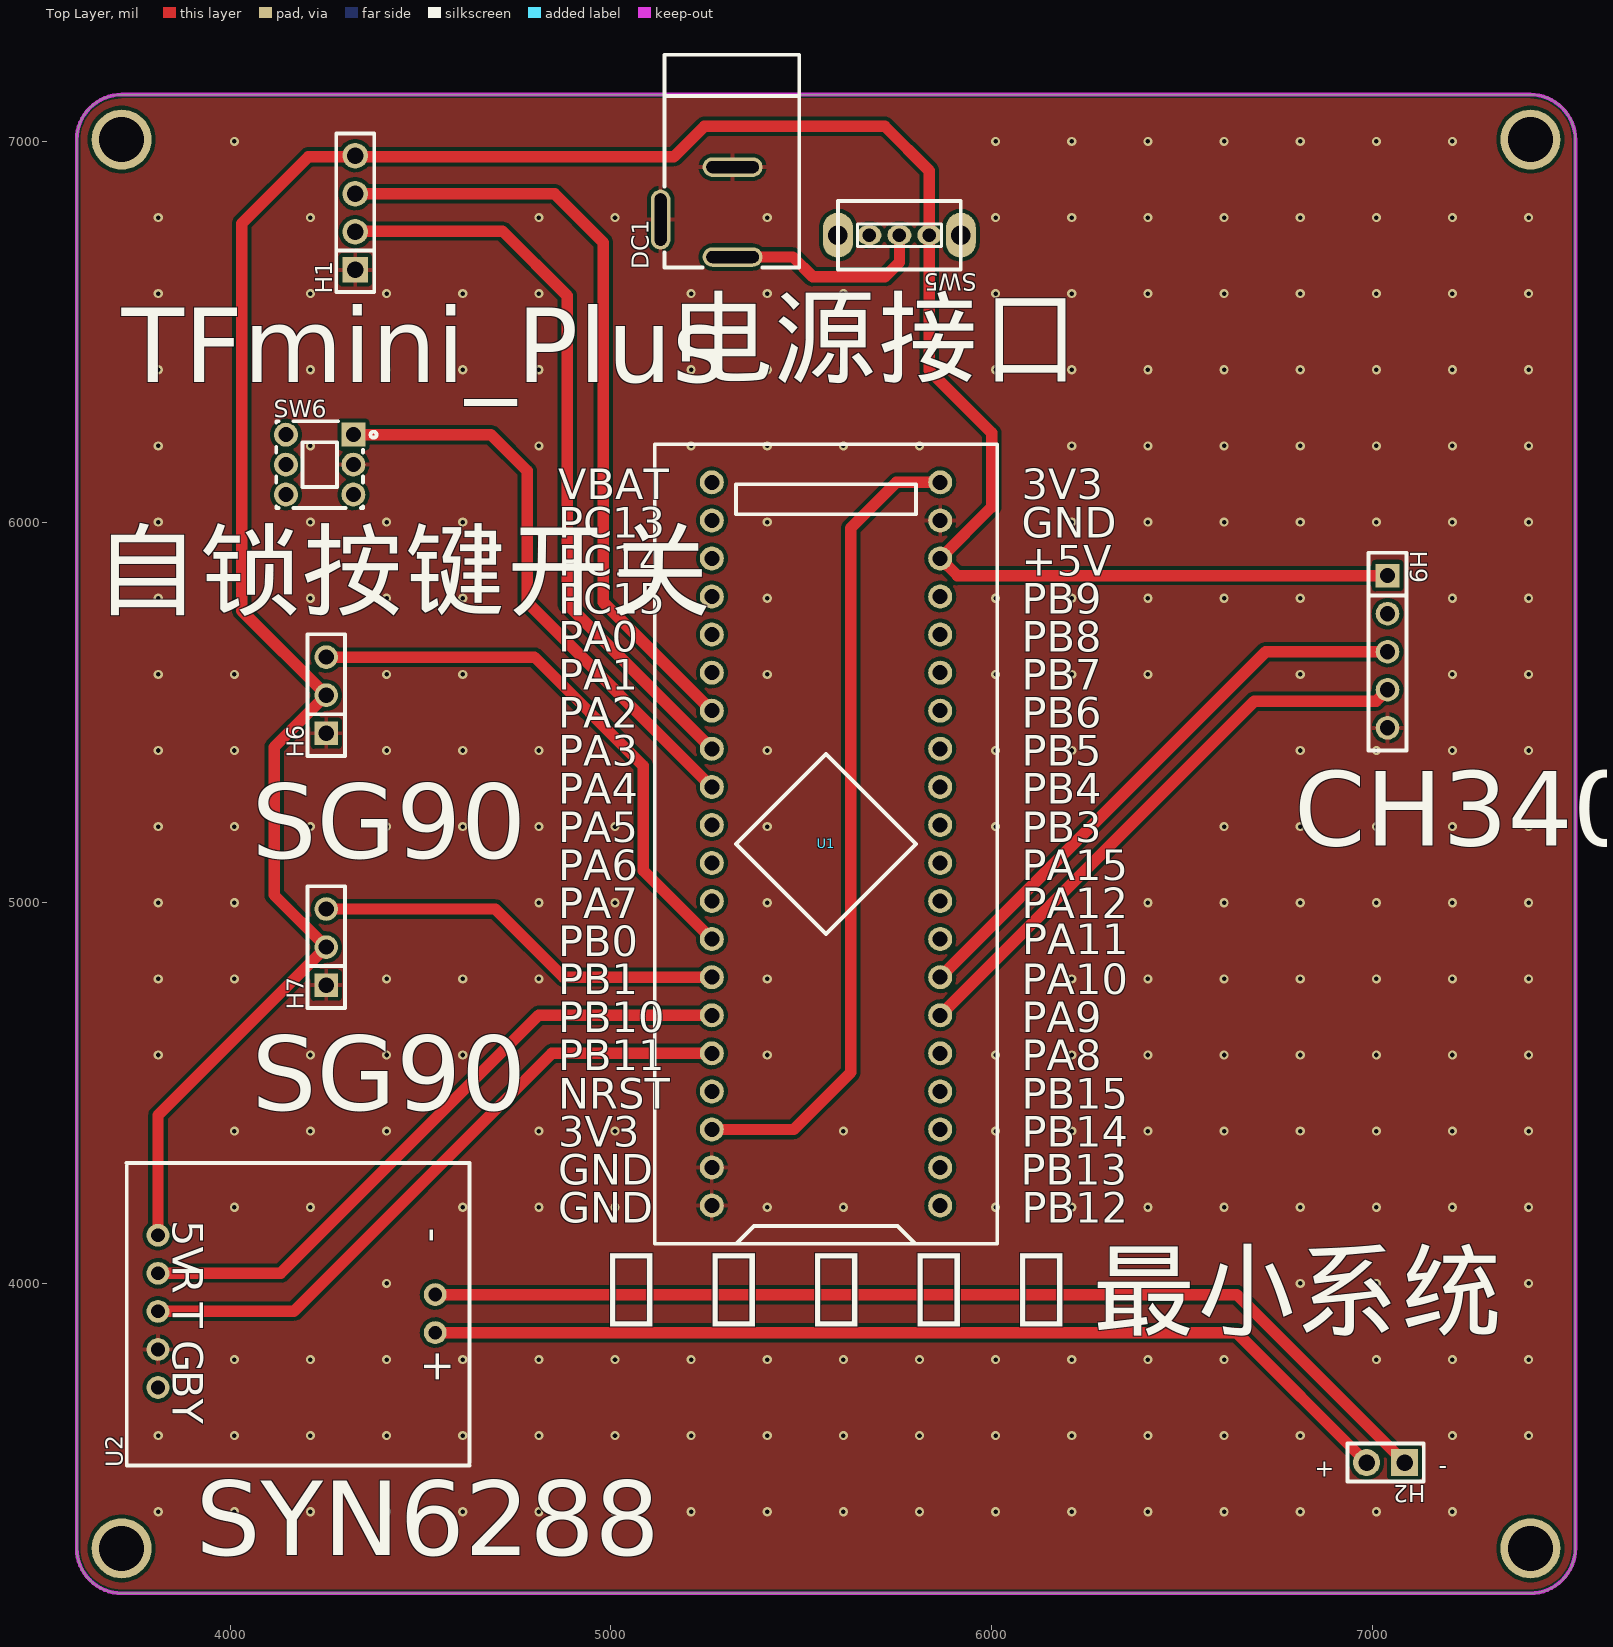
[diagram p0: Top Layer view]
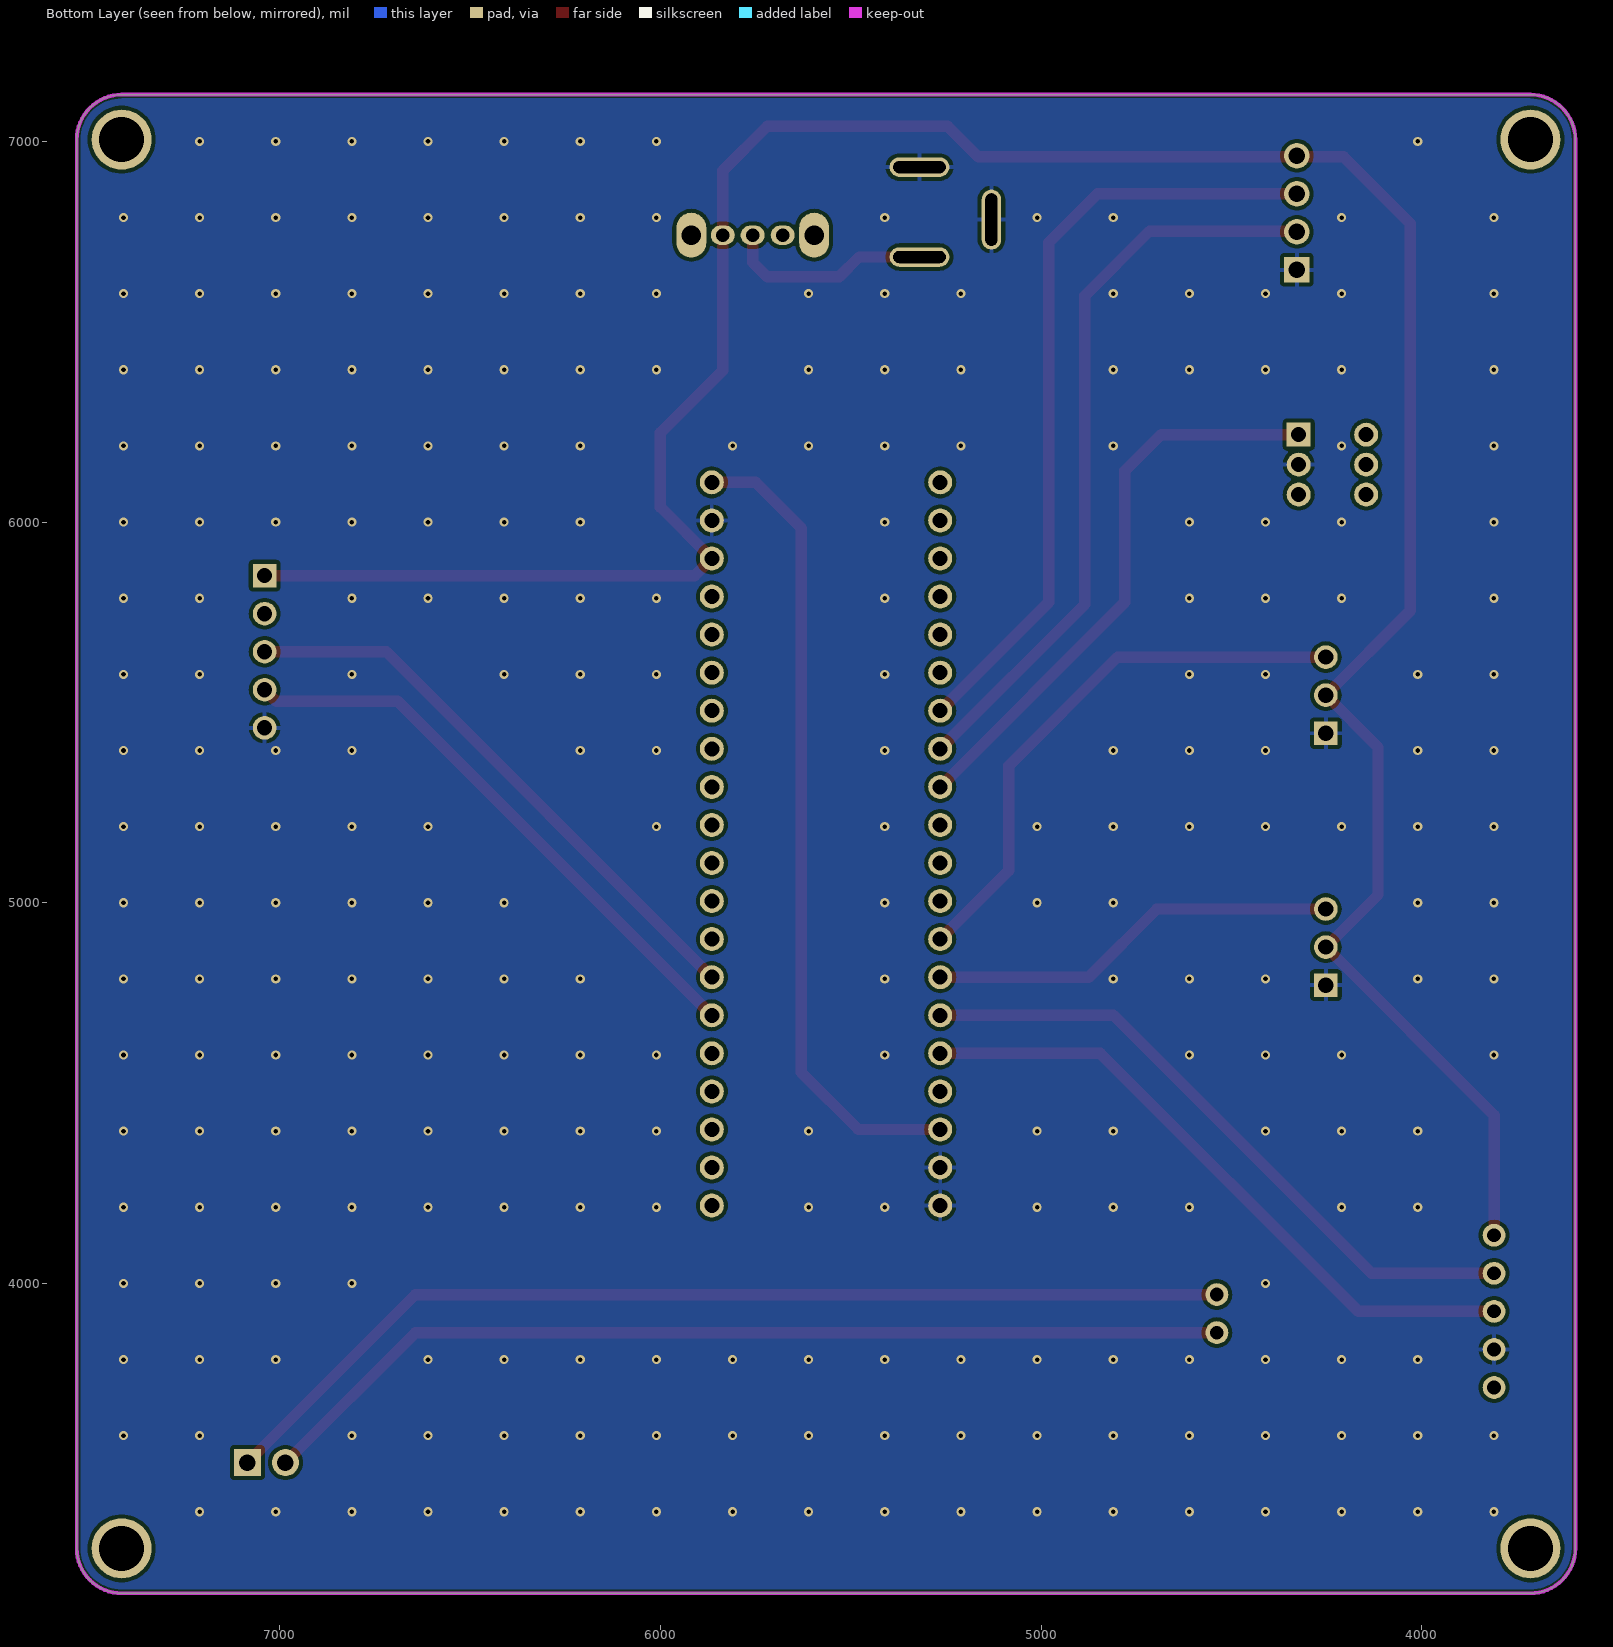
[diagram p1: Bottom Layer view, seen from below]
# Altium PCB MISC51113.pcbdoc
Units mil, origin at the board's own origin, x right, y up, seen from the top; angles counter-clockwise.
Board outline 3937.01 x 3937.01 mil, 2 copper layers (Top Layer, Bottom Layer), stack 62.206 mil thick; 10 components, 40 nets, 82 pads, 252 vias.

## Layer stack, top to bottom
Top Solder Mask Layer: solder mask 0.394, Dk 3.3
Top Layer: signal copper 1.379
Dielectric1: surface 59.449, FR4, Dk 4.5
Bottom Layer: signal copper 1.378
Bottom Solder Mask Layer: solder mask 0.394, Dk 3.3

## Board outline
3714.61,7123.5 ccw(c3714.61,7005.39) 3596.5,7005.39 3596.5,3304.61 ccw(c3714.61,3304.61) 3714.61,3186.5 7415.39,3186.5 ccw(c7415.39,3304.61) 7533.5,3304.61 7533.5,7005.39 ccw(c7415.39,7005.39) 7415.39,7123.5 3714.61,7123.5

## Design rules (kind name [scope] priority, off if disabled: settings)
BoardOutlineClearance copperThickness2oz_1 [All] p2 off: genericclearance=7.99 ignorepadtopadclearanceinfootprint=FALSE except(0: Arc-SplitContinuation Track-SplitContinuation SMDPad-SplitContinuation THPad-SplitContinuation Via-SplitContinuation Fill-SplitContinuation Region-SplitContinuation Poly-SplitContinuation Text-SplitContinuation Hole-SplitContinuation; 5.98: Arc-CutoutEdge Track-CutoutEdge SMDPad-CutoutEdge THPad-CutoutEdge Via-CutoutEdge Text-CutoutEdge; 6.9: Hole-OutlineEdge Hole-CutoutEdge; 10: Poly-OutlineEdge Poly-CutoutEdge; 11.81: Arc-OutlineEdge Track-OutlineEdge SMDPad-OutlineEdge THPad-OutlineEdge Via-OutlineEdge Fill-OutlineEdge Region-OutlineEdge Text-OutlineEdge Fill-CutoutEdge Region-CutoutEdge)
BoardOutlineClearance Plane_innerPlane_1 [All] p4 off: genericclearance=4.02 ignorepadtopadclearanceinfootprint=FALSE except(0: Arc-SplitContinuation Track-SplitContinuation SMDPad-SplitContinuation THPad-SplitContinuation Via-SplitContinuation Fill-SplitContinuation Region-SplitContinuation Poly-SplitContinuation Text-SplitContinuation Hole-SplitContinuation; 5.98: Arc-CutoutEdge Track-CutoutEdge SMDPad-CutoutEdge THPad-CutoutEdge Via-CutoutEdge Text-CutoutEdge; 6.9: Hole-OutlineEdge Hole-CutoutEdge; 10: Poly-OutlineEdge Poly-CutoutEdge; 11.81: Arc-OutlineEdge Track-OutlineEdge SMDPad-OutlineEdge THPad-OutlineEdge Via-OutlineEdge Fill-OutlineEdge Region-OutlineEdge Text-OutlineEdge Fill-CutoutEdge Region-CutoutEdge)
BoardOutlineClearance Copper_copperRegion_1 [All] p6 off: genericclearance=4.02 ignorepadtopadclearanceinfootprint=FALSE except(0: Arc-SplitContinuation Track-SplitContinuation SMDPad-SplitContinuation THPad-SplitContinuation Via-SplitContinuation Fill-SplitContinuation Region-SplitContinuation Poly-SplitContinuation Text-SplitContinuation Hole-SplitContinuation; 5.98: Arc-CutoutEdge Track-CutoutEdge SMDPad-CutoutEdge THPad-CutoutEdge Via-CutoutEdge Text-CutoutEdge; 6.9: Hole-OutlineEdge Hole-CutoutEdge; 10: Poly-OutlineEdge Poly-CutoutEdge; 11.81: Arc-OutlineEdge Track-OutlineEdge SMDPad-OutlineEdge THPad-OutlineEdge Via-OutlineEdge Fill-OutlineEdge Region-OutlineEdge Text-OutlineEdge Fill-CutoutEdge Region-CutoutEdge)
BoardOutlineClearance Copper_copperRegion_copperThickness1oz_1 [All] p8 off: genericclearance=4.02 ignorepadtopadclearanceinfootprint=FALSE except(0: Arc-SplitContinuation Track-SplitContinuation SMDPad-SplitContinuation THPad-SplitContinuation Via-SplitContinuation Fill-SplitContinuation Region-SplitContinuation Poly-SplitContinuation Text-SplitContinuation Hole-SplitContinuation; 5.98: Arc-CutoutEdge Track-CutoutEdge SMDPad-CutoutEdge THPad-CutoutEdge Via-CutoutEdge Text-CutoutEdge; 6.9: Hole-OutlineEdge Hole-CutoutEdge; 10: Poly-OutlineEdge Poly-CutoutEdge; 11.81: Arc-OutlineEdge Track-OutlineEdge SMDPad-OutlineEdge THPad-OutlineEdge Via-OutlineEdge Fill-OutlineEdge Region-OutlineEdge Text-OutlineEdge Fill-CutoutEdge Region-CutoutEdge)
BoardOutlineClearance Copper_copperRegion_Copper_copperRegion_1 [All] p10 off: genericclearance=4.02 ignorepadtopadclearanceinfootprint=FALSE except(0: Arc-SplitContinuation Track-SplitContinuation SMDPad-SplitContinuation THPad-SplitContinuation Via-SplitContinuation Fill-SplitContinuation Region-SplitContinuation Poly-SplitContinuation Text-SplitContinuation Hole-SplitContinuation; 5.98: Arc-CutoutEdge Track-CutoutEdge SMDPad-CutoutEdge THPad-CutoutEdge Via-CutoutEdge Text-CutoutEdge; 6.9: Hole-OutlineEdge Hole-CutoutEdge; 10: Poly-OutlineEdge Poly-CutoutEdge; 11.81: Arc-OutlineEdge Track-OutlineEdge SMDPad-OutlineEdge THPad-OutlineEdge Via-OutlineEdge Fill-OutlineEdge Region-OutlineEdge Text-OutlineEdge Fill-CutoutEdge Region-CutoutEdge)
BoardOutlineClearance copperThickness1oz_1 [All] p12: genericclearance=4.02 ignorepadtopadclearanceinfootprint=FALSE except(0: Arc-SplitContinuation Track-SplitContinuation SMDPad-SplitContinuation THPad-SplitContinuation Via-SplitContinuation Fill-SplitContinuation Region-SplitContinuation Poly-SplitContinuation Text-SplitContinuation Hole-SplitContinuation; 5.98: Arc-CutoutEdge Track-CutoutEdge SMDPad-CutoutEdge THPad-CutoutEdge Via-CutoutEdge Text-CutoutEdge; 6.9: Hole-OutlineEdge Hole-CutoutEdge; 10: Poly-OutlineEdge Poly-CutoutEdge; 11.81: Arc-OutlineEdge Track-OutlineEdge SMDPad-OutlineEdge THPad-OutlineEdge Via-OutlineEdge Fill-OutlineEdge Region-OutlineEdge Text-OutlineEdge Fill-CutoutEdge Region-CutoutEdge)
Clearance copperThickness2oz [All] p1 off: gap=7.99 ignorepadtopadclearanceinfootprint=FALSE except(5.98: SMDPad-Track SMDPad-SMDPad THPad-Track SMDPad-THPad THPad-THPad Track-Via SMDPad-Via THPad-Via Via-Via Fill-SMDPad Region-SMDPad Fill-THPad Region-THPad Fill-Via Region-Via Fill-Fill Fill-Region Region-Region Arc-Track Arc-SMDPad Arc-THPad Arc-Via Fill-Arc Region-Arc Arc-Arc Text-Track SMDPad-Text Text-THPad Text-Via Fill-Text Region-Text Arc-Text Text-Text; 6.9: Hole-Track Hole-SMDPad Hole-THPad Hole-Via Fill-Hole Region-Hole Hole-Arc Hole-Text; 10: Poly-Track Poly-SMDPad Poly-THPad Poly-Via Poly-Fill Poly-Region Poly-Poly Poly-Arc Poly-Text Poly-Hole; 11.81: Fill-Track Region-Track)
Clearance Plane_innerPlane [All] p3 off: gap=4.02 ignorepadtopadclearanceinfootprint=FALSE except(5.98: SMDPad-Track SMDPad-SMDPad THPad-Track SMDPad-THPad THPad-THPad Track-Via SMDPad-Via THPad-Via Via-Via Fill-SMDPad Region-SMDPad Fill-THPad Region-THPad Fill-Via Region-Via Fill-Fill Fill-Region Region-Region Arc-Track Arc-SMDPad Arc-THPad Arc-Via Fill-Arc Region-Arc Arc-Arc Text-Track SMDPad-Text Text-THPad Text-Via Fill-Text Region-Text Arc-Text Text-Text; 6.9: Hole-Track Hole-SMDPad Hole-THPad Hole-Via Fill-Hole Region-Hole Hole-Arc Hole-Text; 10: Poly-Track Poly-SMDPad Poly-THPad Poly-Via Poly-Fill Poly-Region Poly-Poly Poly-Arc Poly-Text Poly-Hole; 11.81: Fill-Track Region-Track)
Clearance Copper_copperRegion [All] p5 off: gap=4.02 ignorepadtopadclearanceinfootprint=FALSE except(5.98: SMDPad-Track SMDPad-SMDPad THPad-Track SMDPad-THPad THPad-THPad Track-Via SMDPad-Via THPad-Via Via-Via Fill-SMDPad Region-SMDPad Fill-THPad Region-THPad Fill-Via Region-Via Fill-Fill Fill-Region Region-Region Arc-Track Arc-SMDPad Arc-THPad Arc-Via Fill-Arc Region-Arc Arc-Arc Text-Track SMDPad-Text Text-THPad Text-Via Fill-Text Region-Text Arc-Text Text-Text; 6.9: Hole-Track Hole-SMDPad Hole-THPad Hole-Via Fill-Hole Region-Hole Hole-Arc Hole-Text; 10: Poly-Track Poly-SMDPad Poly-THPad Poly-Via Poly-Fill Poly-Region Poly-Poly Poly-Arc Poly-Text Poly-Hole; 11.81: Fill-Track Region-Track)
Clearance Copper_copperRegion_copperThickness1oz [All] p7 off: gap=4.02 ignorepadtopadclearanceinfootprint=FALSE except(5.98: SMDPad-Track SMDPad-SMDPad THPad-Track SMDPad-THPad THPad-THPad Track-Via SMDPad-Via THPad-Via Via-Via Fill-SMDPad Region-SMDPad Fill-THPad Region-THPad Fill-Via Region-Via Fill-Fill Fill-Region Region-Region Arc-Track Arc-SMDPad Arc-THPad Arc-Via Fill-Arc Region-Arc Arc-Arc Text-Track SMDPad-Text Text-THPad Text-Via Fill-Text Region-Text Arc-Text Text-Text; 6.9: Hole-Track Hole-SMDPad Hole-THPad Hole-Via Fill-Hole Region-Hole Hole-Arc Hole-Text; 10: Poly-Track Poly-SMDPad Poly-THPad Poly-Via Poly-Fill Poly-Region Poly-Poly Poly-Arc Poly-Text Poly-Hole; 11.81: Fill-Track Region-Track)
Clearance Copper_copperRegion_Copper_copperRegion [All] p9 off: gap=4.02 ignorepadtopadclearanceinfootprint=FALSE except(5.98: SMDPad-Track SMDPad-SMDPad THPad-Track SMDPad-THPad THPad-THPad Track-Via SMDPad-Via THPad-Via Via-Via Fill-SMDPad Region-SMDPad Fill-THPad Region-THPad Fill-Via Region-Via Fill-Fill Fill-Region Region-Region Arc-Track Arc-SMDPad Arc-THPad Arc-Via Fill-Arc Region-Arc Arc-Arc Text-Track SMDPad-Text Text-THPad Text-Via Fill-Text Region-Text Arc-Text Text-Text; 6.9: Hole-Track Hole-SMDPad Hole-THPad Hole-Via Fill-Hole Region-Hole Hole-Arc Hole-Text; 10: Poly-Track Poly-SMDPad Poly-THPad Poly-Via Poly-Fill Poly-Region Poly-Poly Poly-Arc Poly-Text Poly-Hole; 11.81: Fill-Track Region-Track)
Clearance copperThickness1oz [All] p11: gap=4.02 ignorepadtopadclearanceinfootprint=FALSE except(5.98: SMDPad-Track SMDPad-SMDPad THPad-Track SMDPad-THPad THPad-THPad Track-Via SMDPad-Via THPad-Via Via-Via Fill-SMDPad Region-SMDPad Fill-THPad Region-THPad Fill-Via Region-Via Fill-Fill Fill-Region Region-Region Arc-Track Arc-SMDPad Arc-THPad Arc-Via Fill-Arc Region-Arc Arc-Arc Text-Track SMDPad-Text Text-THPad Text-Via Fill-Text Region-Text Arc-Text Text-Text; 6.9: Hole-Track Hole-SMDPad Hole-THPad Hole-Via Fill-Hole Region-Hole Hole-Arc Hole-Text; 10: Poly-Track Poly-SMDPad Poly-THPad Poly-Via Poly-Fill Poly-Region Poly-Poly Poly-Arc Poly-Text Poly-Hole; 11.81: Fill-Track Region-Track)
DiffPairsRouting differentialPair [All] p1: maxlimit=6 minlimit=6 mostfreqgap=6 toplayer_minwidth=5 toplayer_prefwidth=10 toplayer_maxwidth=100 toplayer_mingap=6 toplayer_prefgap=6 toplayer_maxgap=6 bottomlayer_minwidth=5 bottomlayer_prefwidth=10 bottomlayer_maxwidth=100 bottomlayer_mingap=6 bottomlayer_prefgap=6 bottomlayer_maxgap=6 maxuncoupledlength=10
HoleToHoleClearance otherClearance [All] p1: gap=11.81 allowstackedmicrovias=TRUE
Length netLength [All] p1: minlimit=0 maxlimit=0
PasteMaskExpansion pasteMaskExpansion [All] p1: expansion=0
PlaneConnect innerPlane [All] p1: planeconnectstyle=Relief reliefexpansion=20 reliefentries=4 reliefconductorwidth=10 reliefairgap=10
PolygonConnect copperRegion_copperThickness1oz [All] p1 off: connectstyle=Relief reliefconductorwidth=10 reliefentries=4 polygonreliefangle="90 Angle" airgapwidth=10 via.connectstyle=Relief via.reliefconductorwidth=10 via.reliefentries=4 via.polygonreliefangle="90 Angle" via.airgapwidth=10
PolygonConnect copperRegion_Copper_copperRegion [All] p2 off: connectstyle=Relief reliefconductorwidth=10 reliefentries=4 polygonreliefangle="90 Angle" airgapwidth=10 via.connectstyle=Relief via.reliefconductorwidth=10 via.reliefentries=4 via.polygonreliefangle="90 Angle" via.airgapwidth=10
PolygonConnect copperRegion [All] p3: connectstyle=Relief reliefconductorwidth=10 reliefentries=4 polygonreliefangle="90 Angle" airgapwidth=10 via.connectstyle=Relief via.reliefconductorwidth=10 via.reliefentries=4 via.polygonreliefangle="90 Angle" via.airgapwidth=10
RoutingVias viaSize [All] p1: holewidth=12.01 width=24.02 viastyle="Through Hole" minholewidth=11.81 minwidth=19.68 maxholewidth=248.03 maxwidth=393.7
SolderMaskExpansion solderMaskExpansion [IsVia] p1: expansion=-1000 istentingtop=TRUE
SolderMaskExpansion solderMaskExpansion [All] p2: expansion=2 istentingtop=FALSE
Width copperThickness2oz_2 [All] p1 off: maxlimit=100 minlimit=8 preferedwidth=10
Width copperThickness1oz_2 [All] p2: maxlimit=100 minlimit=5 preferedwidth=10

## Components (designator, comment, footprint, x,y, rotation, side; value= is the part's Value field where it differs from the comment)
DC1 "" DC-2.0 5330,6820 r90 top
H1 "" HDR-TH_4P-P2.54-V-F 4328.17,6813.05 r90 top
H2 "" HDR-TH_2P-P2.54-V-M-1 7035,3530 r180 top
H6 "" HDR-TH_3P-P2.54-V-F 4251.93,5546 r90 top
H7 "" HDR-TH_3P-P2.54-V-F 4251.93,4884.13 r90 top
H9 "" HDR-TH_5P-P2.54-V-F 7040,5660 r270 top
SW5 "" 拨动开关 5762.9,6754.15 r180 top
SW6 "TK-6580-1" SW-TH_TK-6580-1 4234.67,6151.45 r0 top
U1 "STM32F103C8T6-Card" CONN-TH_L53.3-W22.9_STM32F103C8T6-CARD 5565,5155 r90 top
U2 "SYN6288" SYN6288 4125,3950 r90 top

## Footprints (in the part's own frame and the unit in brackets; to place one, negate y for a bottom-side part, rotate by r counter-clockwise, add the part's x,y. Pads: shape width x height; smd on the part's side, far side on the other; paste and mask are expansions set on the pad)
CONN-TH_L53.3-W22.9_STM32F103C8T6-CARD [mm]
  round 1.6 hole 1: 1(-24.13,-7.62) 2(-21.59,-7.62) 3(-19.05,-7.62) 4(-16.51,-7.62) 5(-13.97,-7.62) 6(-11.43,-7.62) 7(-8.89,-7.62) 8(-6.35,-7.62) 9(-3.81,-7.62) 10(-1.27,-7.62) 11(1.27,-7.62) 12(3.81,-7.62) 13(6.35,-7.62) 14(8.89,-7.62) 15(11.43,-7.62) 16(13.97,-7.62) 17(16.51,-7.62) 18(19.05,-7.62) 19(21.59,-7.62) 20(24.13,-7.62) 21(24.13,7.62) 22(21.59,7.62) 23(19.05,7.62) 24(16.51,7.62) 25(13.97,7.62) 26(11.43,7.62) 27(8.89,7.62) 28(6.35,7.62) 29(3.81,7.62) 30(1.27,7.62) 31(-1.27,7.62) 32(-3.81,7.62) 33(-6.35,7.62) 34(-8.89,7.62) 35(-11.43,7.62) 36(-13.97,7.62) 37(-16.51,7.62) 38(-19.05,7.62) 39(-21.59,7.62) 40(-24.13,7.62)
  silkscreen extent -26.67,-11.43 26.67,11.43
DC-2.0 [mil]
  oval 157.5x51.2 hole 31.5 slot 137.8 at 0 deg paste+0 mask+2: 2(-24.7,199.5)
  oval 51.2x157.5 hole 31.5 slot 137.8 at 90 deg paste+0 mask+2: 3(113.1,10.5) 4(-123.1,10.5)
  silkscreen extent -151,-165 408,190
HDR-TH_2P-P2.54-V-M-1 [mm]
  rect 1.8x1.8 hole 1.1: 1(-1.27,0)
  round 1.8 hole 1.1: 2(1.27,0)
  silkscreen extent -2.54,-1.27 2.54,1.27
HDR-TH_3P-P2.54-V-F [mil]
  rect 62x62 hole 40.16: 1(-100,0)
  round 62 hole 40.16: 2(0,0) 3(100,0)
  silkscreen extent -160,-49 160,49
HDR-TH_4P-P2.54-V-F [mm]
  rect 1.7x1.7 hole 1.1: 1(-3.81,0)
  round 1.7 hole 1.1: 2(-1.27,0) 3(1.27,0) 4(3.81,0)
  silkscreen extent -5.29,-1.27 5.29,1.27
HDR-TH_5P-P2.54-V-F [mil]
  rect 62x62 hole 40.16: 1(-200,0)
  round 62 hole 40.16: 2(-100,0) 3(0,0) 4(100,0) 5(200,0)
  silkscreen extent -260,-50 260,50
SW-TH_TK-6580-1 [mm]
  rect 1.6x1.6 hole 1: 1(2.25,2)
  round 1.6 hole 1: 2(2.25,0) 3(2.25,-2) 4(-2.25,2) 5(-2.25,0) 6(-2.25,-2)
  silkscreen extent -2.9,-2.9 3.8,2.9
SYN6288 [mil]
  round 60 hole 36 paste+0 mask+2: 1(177.16,314.96) 2(77.16,314.96) 3(-22.84,314.96) 4(-122.84,314.96) 5(-222.84,314.96) 6(21.26,-413.39) 7(-78.74,-413.39)
  silkscreen extent -428,-504 367,398
拨动开关 [mil]
  oval 63x51.2 hole 35.4 paste+0 mask+2: 1(-73.4,0) 2(5,0) 3(84,0)
  oval 78.7x118.1 hole 51.2 paste+0 mask+2: 4(166.7,0) 5(-156.1,0)
  silkscreen extent -156,-90 167,90

## Free pads (board coordinates)
  round 157.48 hole 118.11: 1(3714.61,7005.39) 1(3714.61,3304.61) 1(7415.39,7005.39) 1(7415.39,3304.61)

## Via types
v1: diameter 24.02, hole 12, Top Layer to Bottom Layer, 252 vias

## Nets (pads, with @x,y where several pads share a name; then routed paths per layer and width w, separated by ;. In a path a pad name is that pad's centre, name@x,y a point inside that pad or via, vN(x,y) a via of type N, cw(c..) or ccw(c..) an arc to the next point about the centre after c; other vN are vias at no path point)
$1N17118: DC1.4 SW5.2 | length 546.9
  Top Layer w30: DC1.4 5478.1,6696.9 5530,6645 5720,6645 5757.9,6682.9 SW5.2
$1N17262: H2.1 U2.6 | length 2729.4
  Top Layer w30: U2.6 6643.74,3971.26 H2.1
$1N17263: H2.2 U2.7 | length 2588
  Top Layer w30: U2.7 6643.74,3871.26 H2.2
+5V: H1.4 H6.2 H7.2 H9.1 SW5.1 U1.18 U2.1 | length 7342.4
  Top Layer w30: U2.1 3810.04,4442.25 H7.2 4115,5021.06 4115,5409.07 H6.2 4030,5767.92 4030,6785 4205,6960 5165,6960 5245,7040 5720,7040 5836.3,6923.7 SW5.1 5836.3,6398.7 6000,6235 6000,6040 U1.18 5910,5860 H9.1
GND: DC1.2 DC1.3 H1.1 H6.1 H7.1 H9.5 SW6.2 U1.19 U1.39 U1.40 U2.4
  other v1: 3810.6,3400.6 4010.6,3400.6 4210.6,3400.6 4410.6,3400.6 4610.6,3400.6 4810.6,3400.6 5010.6,3400.6 5210.6,3400.6 5410.6,3400.6 5610.6,3400.6 5810.6,3400.6 6010.6,3400.6 6210.6,3400.6 6410.6,3400.6 6610.6,3400.6 6810.6,3400.6 7010.6,3400.6 7210.6,3400.6 3810.6,3600.6 4010.6,3600.6 4210.6,3600.6 4410.6,3600.6 4610.6,3600.6 4810.6,3600.6 5010.6,3600.6 5210.6,3600.6 5410.6,3600.6 5610.6,3600.6 5810.6,3600.6 6010.6,3600.6 6210.6,3600.6 6410.6,3600.6 6610.6,3600.6 6810.6,3600.6 7210.6,3600.6 7410.6,3600.6 4010.6,3800.6 4210.6,3800.6 4410.6,3800.6 4610.6,3800.6 4810.6,3800.6 5010.6,3800.6 5210.6,3800.6 5410.6,3800.6 5610.6,3800.6 5810.6,3800.6 6010.6,3800.6 6210.6,3800.6 6410.6,3800.6 6610.6,3800.6 7010.6,3800.6 7210.6,3800.6 7410.6,3800.6 4410.6,4000.6 6810.6,4000.6 7010.6,4000.6 7210.6,4000.6 7410.6,4000.6 4010.6,4200.6 4210.6,4200.6 4610.6,4200.6 4810.6,4200.6 5010.6,4200.6 5410.6,4200.6 5610.6,4200.6 6010.6,4200.6 6210.6,4200.6 6410.6,4200.6 6610.6,4200.6 6810.6,4200.6 7010.6,4200.6 7210.6,4200.6 7410.6,4200.6 4010.6,4400.6 4210.6,4400.6 4410.6,4400.6 4810.6,4400.6 5010.6,4400.6 5610.6,4400.6 6010.6,4400.6 6210.6,4400.6 6410.6,4400.6 6610.6,4400.6 6810.6,4400.6 7010.6,4400.6 7210.6,4400.6 7410.6,4400.6 3810.6,4600.6 4210.6,4600.6 4410.6,4600.6 4610.6,4600.6 5410.6,4600.6 6010.6,4600.6 6210.6,4600.6 6410.6,4600.6 6610.6,4600.6 6810.6,4600.6 7010.6,4600.6 7210.6,4600.6 7410.6,4600.6 3810.6,4800.6 4010.6,4800.6 4410.6,4800.6 4610.6,4800.6 4810.6,4800.6 5410.6,4800.6 6210.6,4800.6 6410.6,4800.6 6610.6,4800.6 6810.6,4800.6 7010.6,4800.6 7210.6,4800.6 7410.6,4800.6 3810.6,5000.6 4010.6,5000.6 4810.6,5000.6 5010.6,5000.6 5410.6,5000.6 6410.6,5000.6 6610.6,5000.6 6810.6,5000.6 7010.6,5000.6 7210.6,5000.6 7410.6,5000.6 3810.6,5200.6 4010.6,5200.6 4210.6,5200.6 4410.6,5200.6 4610.6,5200.6 4810.6,5200.6 5010.6,5200.6 5410.6,5200.6 6010.6,5200.6 6610.6,5200.6 6810.6,5200.6 7010.6,5200.6 7210.6,5200.6 7410.6,5200.6 3810.6,5400.6 4010.6,5400.6 4410.6,5400.6 4610.6,5400.6 4810.6,5400.6 5410.6,5400.6 6010.6,5400.6 6210.6,5400.6 6810.6,5400.6 7010.6,5400.6 7210.6,5400.6 7410.6,5400.6 3810.6,5600.6 4010.6,5600.6 4410.6,5600.6 4610.6,5600.6 5410.6,5600.6 6010.6,5600.6 6210.6,5600.6 6410.6,5600.6 6810.6,5600.6 7210.6,5600.6 7410.6,5600.6 3810.6,5800.6 4210.6,5800.6 4410.6,5800.6 4610.6,5800.6 5410.6,5800.6 6010.6,5800.6 6210.6,5800.6 6410.6,5800.6 6610.6,5800.6 6810.6,5800.6 7210.6,5800.6 7410.6,5800.6 3810.6,6000.6 4210.6,6000.6 4410.6,6000.6 4610.6,6000.6 5410.6,6000.6 6210.6,6000.6 6410.6,6000.6 6610.6,6000.6 6810.6,6000.6 7010.6,6000.6 7210.6,6000.6 7410.6,6000.6 3810.6,6200.6 4210.6,6200.6 4810.6,6200.6 5210.6,6200.6 5410.6,6200.6 5610.6,6200.6 5810.6,6200.6 6210.6,6200.6 6410.6,6200.6 6610.6,6200.6 6810.6,6200.6 7010.6,6200.6 7210.6,6200.6 7410.6,6200.6 3810.6,6400.6 4210.6,6400.6 4410.6,6400.6 4610.6,6400.6 4810.6,6400.6 5210.6,6400.6 5410.6,6400.6 5610.6,6400.6 6010.6,6400.6 6210.6,6400.6 6410.6,6400.6 6610.6,6400.6 6810.6,6400.6 7010.6,6400.6 7210.6,6400.6 7410.6,6400.6 3810.6,6600.6 4210.6,6600.6 4410.6,6600.6 4610.6,6600.6 4810.6,6600.6 5210.6,6600.6 5410.6,6600.6 5610.6,6600.6 6010.6,6600.6 6210.6,6600.6 6410.6,6600.6 6610.6,6600.6 6810.6,6600.6 7010.6,6600.6 7210.6,6600.6 7410.6,6600.6 3810.6,6800.6 4210.6,6800.6 4810.6,6800.6 5010.6,6800.6 5410.6,6800.6 6010.6,6800.6 6210.6,6800.6 6410.6,6800.6 6610.6,6800.6 6810.6,6800.6 7010.6,6800.6 7210.6,6800.6 7410.6,6800.6 4010.6,7000.6 6010.6,7000.6 6210.6,7000.6 6410.6,7000.6 6610.6,7000.6 6810.6,7000.6 7010.6,7000.6 7210.6,7000.6
NRST: U1.37
PA0: U1.25
PA1: U1.26
PA2: H1.3 U1.27 | length 2055.4
  Top Layer w30: H1.3@4325.74,6863.16 4851.84,6863.16 4980,6735 4980,5790 U1.27
PA3: H1.2 U1.28 | length 1975.5
  Top Layer w30: H1.2 4330.12,6765 4715,6765 4885,6595 4885,5785 U1.28
PA4: SW6.1 U1.29 | length 1527.1
  Top Layer w30: SW6.1 4684.81,6230.19 4780,6135 4780,5790 U1.29
PA5: U1.30
PA6: U1.31
PA7: U1.32
PA8: U1.5
PA9: H9.4 U1.6 | length 1529.2
  Top Layer w30: U1.6 6690,5530 7010,5530 H9.4
PA10: H9.3 U1.7 | length 1529.2
  Top Layer w30: U1.7 6720,5660 H9.3
PA11: U1.8
PA12: U1.9
PA15: U1.10
PB0: H6.3 U1.33 | length 1481.1
  Top Layer w30: H6.3 4799,5646 5085,5360 5085,5085 U1.33
PB1: H7.3 U1.34 | length 1087.3
  Top Layer w30: H7.3 4695.87,4984.13 4875,4805 U1.34
PB3: U1.11
PB4: U1.12
PB5: U1.13
PB6: U1.14
PB7: U1.15
PB8: U1.16
PB9: U1.17
PB10: U1.35 U2.2 | length 1735.7
  Top Layer w30: U2.2 4132.17,4027.17 4810,4705 U1.35
PB11: U1.36 U2.3 | length 1735.7
  Top Layer w30: U2.3 4167.17,3927.17 4845,4605 U1.36
PB12: U1.1
PB13: U1.2
PB14: U1.3
PB15: U1.4
PC13: U1.22
PC14: U1.23
PC15: U1.24
VBAT: U1.21
VCC: U1.20 U1.38 | length 2141.8
  Top Layer w30: U1.38 5480,4405 5630,4555 5630,5985 5750,6105 U1.20
pads on no net: H9.2 SW5.3 SW5.4 SW5.5 SW6.3 SW6.4 SW6.5 SW6.6 U2.5

## Polygon pours and split planes (outlines as drawn)
GND on Bottom Layer (solid, remove dead copper, pour order 2): 3525,7245 3525,3080 7700,3080 7700,7245
GND on Top Layer (solid, remove dead copper, pour order 2): 3000,7415 3000,3000 7930,3000 7930,7415

## Keep-outs
Board Outline Layer:
  the board outline again, w10

## Silkscreen, mask and mechanical layers (free items; w line width, h text height)
Top Silkscreen Layer:
  text "电源接口" at 5160,6390 h196.85
  text "TFmini_Plus" at 3715.21,6367.37 h196.85
  text "VBAT" at 4860.95,6060 h80
  text "3V3" at 6079.16,6060 h80
  text "PC13" at 4860.95,5960 h80
  text "GND" at 6079.16,5960 h80
  text "PC14" at 4860.95,5860 h80
  text "+5V" at 6079.16,5860 h80
  text "自锁按键开关" at 3648.85,5779.55 h196.85
  text "PC15" at 4860.95,5760 h80
  text "PB9" at 6079.16,5760 h80
  text "PA0" at 4860.95,5660 h80
  text "PB8" at 6079.16,5660 h80
  text "PA1" at 4860.95,5560 h80
  text "PB7" at 6079.16,5560 h80
  text "PA2" at 4860.95,5460 h80
  text "PB6" at 6079.16,5460 h80
  text "PA3" at 4860.95,5360 h80
  text "PB5" at 6079.16,5360 h80
  text "PA4" at 4860.95,5260 h80
  text "PB4" at 6079.16,5260 h80
  text "PA5" at 4860.95,5160 h80
  text "PB3" at 6079.16,5160 h80
  text "CH340" at 6795,5150 h196.85
  text "SG90" at 4055.97,5117.39 h196.85
  text "PA6" at 4860.95,5060 h80
  text "PA15" at 6079.16,5060 h80
  text "PA7" at 4860.95,4960 h80
  text "PA12" at 6079.16,4960 h80
  text "PA11" at 6080.95,4865 h80
  text "PB0" at 4860.95,4860 h80
  text "PB1" at 4860.95,4760 h80
  text "PA10" at 6079.16,4760 h80
  text "PB10" at 4860.95,4660 h80
  text "PA9" at 6079.16,4660 h80
  text "PB11" at 4860.95,4560 h80
  text "PA8" at 6079.16,4560 h80
  text "NRST" at 4860.95,4460 h80
  text "PB15" at 6079.16,4460 h80
  text "SG90" at 4055.97,4455.52 h196.85
  text "3V3" at 4860.95,4360 h80
  text "PB14" at 6079.16,4360 h80
  text "GND" at 4860.95,4260 h80
  text "PB13" at 6075.95,4260 h80
  text "GND" at 4860.95,4160 h80
  text "PB12" at 6079.16,4160 h80
  text "STM32最小系统" at 4919.45,3886.57 h196.85
  text "-" at 7175,3500 h45
  text "+" at 6849,3492.5 h45
  text "SYN6288" at 3909.08,3286.57 h196.85